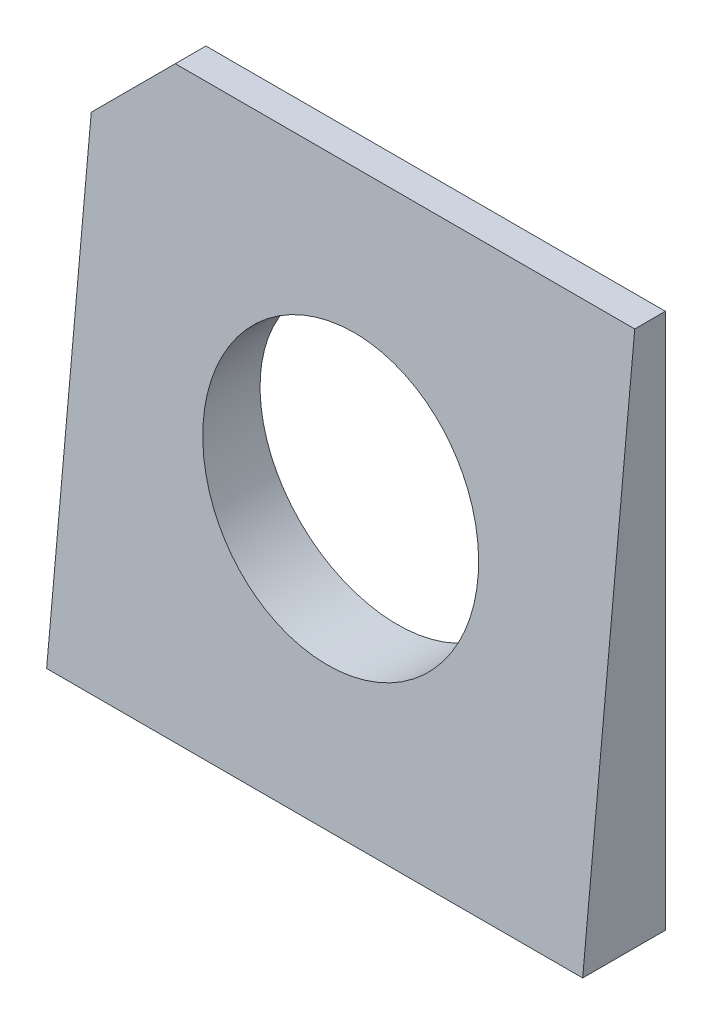
from build123d import *

# Parameters (mm, degrees)
SKETCH1_W          = 35
SKETCH1_H          = 35
SKETCH1_R          = 8.965
BOSS_EXTRUDE_DEPTH = 5.4
SKETCH2_OUTSIDE_W  = 17.358
SKETCH2_OUTSIDE_H  = 46.958
CUT_EXTRUDE1_DEPTH = 35
CUT_EXTRUDE2_DEPTH = 26.331008665


with BuildPart() as part:
    # Sketch1 → Boss-Extrude (new body)
    with BuildSketch(Plane.XY):
        Rectangle(SKETCH1_W, SKETCH1_H)
        with Locations(Location((0, 0, 0), (0, 0, 180))):
            Circle(SKETCH1_R, mode=Mode.SUBTRACT)
    extrude(amount=BOSS_EXTRUDE_DEPTH)

    # Sketch2 outside → Cut-Extrude1 (cut)
    with BuildSketch(Plane(origin=(17.5, 0, 0), x_dir=(0, 0, -1), z_dir=(1, 0, 0))):
        with Locations((-2.7, 0)):
            Rectangle(SKETCH2_OUTSIDE_W, SKETCH2_OUTSIDE_H)
        Polygon((-5.4, -17.5), (-2, 17.5), (0, 17.5), (0, -17.5), align=None, mode=Mode.SUBTRACT)
    extrude(amount=-CUT_EXTRUDE1_DEPTH, mode=Mode.SUBTRACT)

    # Sketch3 → Cut-Extrude2 (cut, through all)
    with BuildSketch(Plane(origin=(0, 0, 0), x_dir=(-1, 0, 0), z_dir=(0, 0, -1))):
        Polygon((12.5, 17.5), (17.5, 12.5), (17.5, 17.5), align=None)
    extrude(amount=-CUT_EXTRUDE2_DEPTH, mode=Mode.SUBTRACT)


solid = part.part
